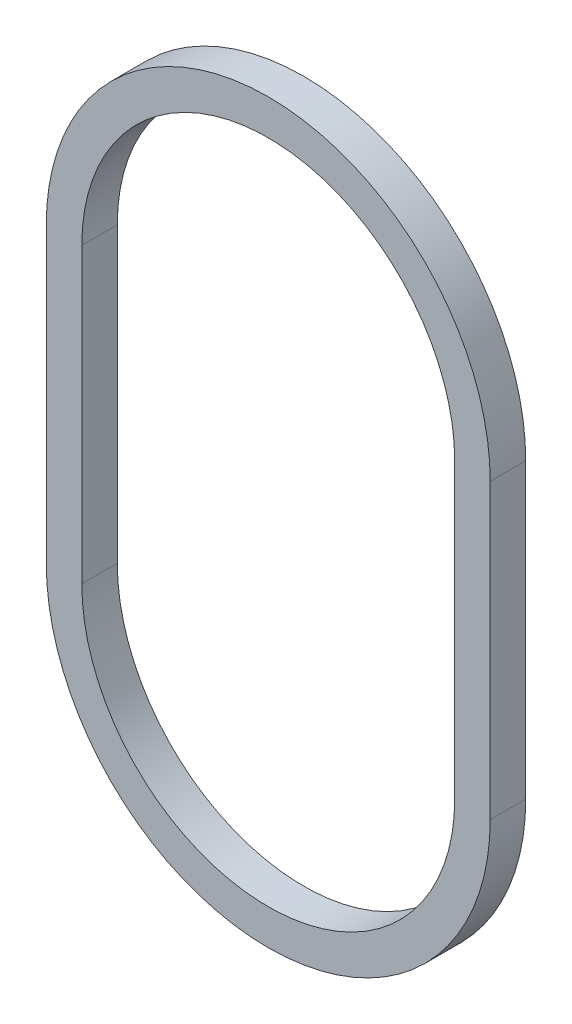
from build123d import *

# Parameters (mm, degrees)
EXTRUDE_1_DEPTH = 4


with BuildPart() as part:
    # 草图1 → 凸台-拉伸1 (new body)
    with BuildSketch(Plane.XY):
        with BuildLine():
            Line((-25, 16.5), (-25, -16.5))
            ThreePointArc((-25, -16.5), (0, -41.5), (25, -16.5))
            Line((25, -16.5), (25, 16.5))
            ThreePointArc((25, 16.5), (0, 41.5), (-25, 16.5))
        make_face()
        with BuildLine():
            Line((-21, 16.5), (-21, -16.5))
            ThreePointArc((-21, -16.5), (0, -37.5), (21, -16.5))
            Line((21, -16.5), (21, 16.5))
            ThreePointArc((21, 16.5), (0, 37.5), (-21, 16.5))
        make_face(mode=Mode.SUBTRACT)
    extrude(amount=EXTRUDE_1_DEPTH)


solid = part.part
